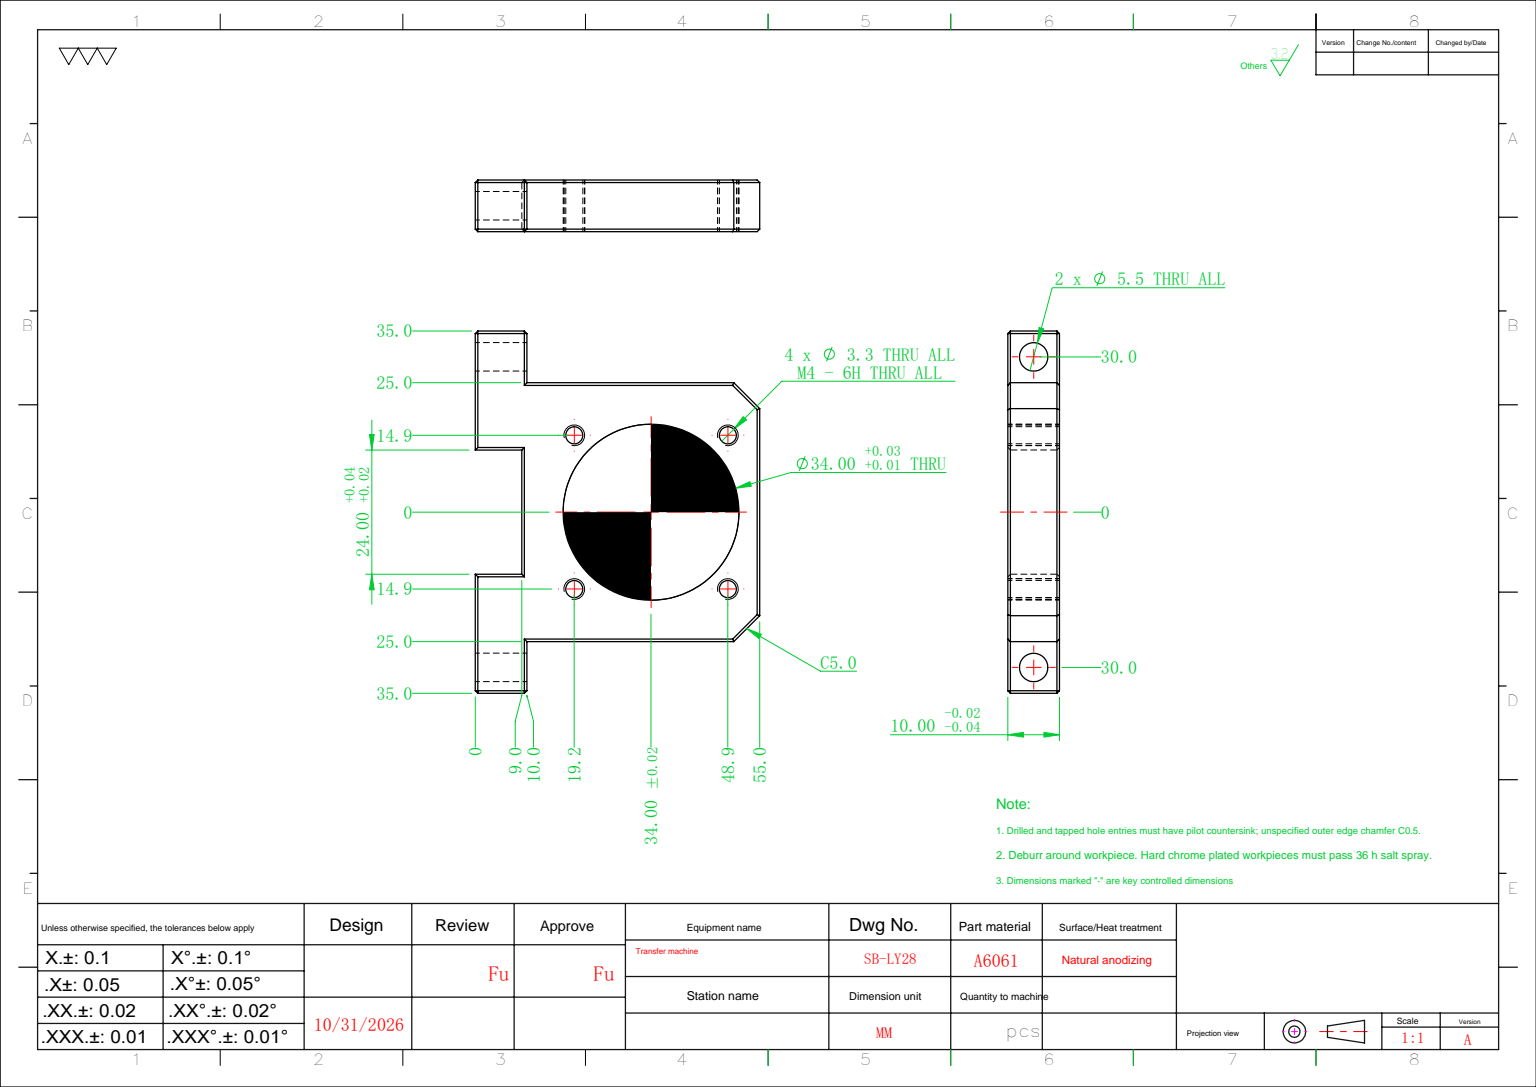
SolidWorks part; units mm, degrees
ref_plane "前视基准面" through (0, 0, 0) normal (0, 0, 1) x (1, 0, 0)
ref_plane "上视基准面" through (0, 0, 0) normal (0, 1, 0) x (1, 0, 0)
ref_plane "右视基准面" through (0, 0, 0) normal (1, 0, 0) x (0, 0, -1)
sketch "草图1" plane through (0, 0, 0) normal (0, 0, 1) x (1, 0, 0)
  line L1 (-35, -27.5) -> (35, -27.5)
  line L2 (-35, -27.5) -> (-35, 27.5)
  line L3 (-35, 27.5) -> (35, 27.5)
  line L4 (35, -27.5) -> (35, 27.5)
  line L5 (-35, -27.5) -> (35, 27.5) construction
  line L6 (-35, 27.5) -> (35, -27.5) construction
  point P0 (0, 0)
  dimension "D1" = 70
  dimension "D2" = 55
extrude "凸台-拉伸1" add sketch "草图1" along normal blind 10
sketch "草图2" plane through (0, 0, 10) normal (0, 0, 1) x (1, 0, 0)
  line L0 (0, 0) -> (0, -35.8295) construction
  line L1 (-35, -27.5) -> (-25, -27.5)
  line L2 (-35, -27.5) -> (-35, 17.5)
  line L3 (-35, 17.5) -> (-25, 17.5)
  line L4 (-25, -27.5) -> (-25, 17.5)
  line L5 (25, -27.5) -> (25, 17.5)
  line L6 (35, 17.5) -> (25, 17.5)
  line L7 (35, -27.5) -> (35, 17.5)
  line L8 (35, -27.5) -> (25, -27.5)
  line L9 (35, 27.5) -> (-35, 27.5) construction
  dimension "D1" = 10
  dimension "D2" = 10
extrude "切除-拉伸1" cut sketch "草图2" against normal through all
sketch "草图3" plane through (0, 0, 0) normal (0, 0, -1) x (-1, 0, 0)
  line L0 (0, 0) -> (0, -40.7468) construction
  line L1 (-35, 27.5) -> (35, 27.5) construction
  circle A0 centre (0, -6.5) radius 17
  dimension "D1" = 34
  dimension "D2" = 34
extrude "切除-拉伸2" cut sketch "草图3" against normal through all
hole_wizard "M4 螺纹孔2" positions "草图8" profile "草图9" tap size "M4" standard "ISO" end condition through all
sketch "草图8" plane through (0, 0, 10) normal (0, 0, 1) x (1, 0, 0)
  line L0 (0, -6.5) -> (0, -34.3856) construction
  line L3 (0, -6.5) -> (-29.4307, -6.5) construction
  point P0 (14.85, -21.35)
  point P2 (-14.85, -21.35)
  point P4 (-14.85, 8.35)
  point P6 (14.85, 8.35)
  dimension "D1" = 29.7
  dimension "D2" = 29.7
sketch "草图9" plane through (14.85, -21.35, 10) normal (1, 0, 0) x (0, -1, 0)
  line L0 (0, 0) -> (0, 10)
  line L1 (0, 10) -> (1.65, 10)
  line L2 (1.65, 10) -> (1.65, 0)
  line L5 (1.65, 0) -> (0, 0)
  line L11 (0, -6.35) -> (0, 107.95) construction
  dimension "通孔螺纹孔钻头直径" = 3.3
  dimension "通孔螺纹孔钻头深度" = 10
cosmetic thread "孔螺蚊线5" parameters "D2"=4
cosmetic thread "孔螺蚊线6" parameters "D2"=4
cosmetic thread "孔螺蚊线7" parameters "D2"=4
cosmetic thread "孔螺蚊线8" parameters "D2"=4
hole_wizard "Ø5.5 (5.5) 直径孔1" positions "草图10" profile "草图11" hole size "Ø5.5" standard "ISO" end condition through all
sketch "草图10" plane through (0, 17.5, 0) normal (0, -1, 0) x (-1, 0, 0)
  line L0 (35, -5) -> (-35, -5) construction
  line L1 (35, 0) -> (35, -10) construction
  line L2 (-35, 0) -> (-35, -10) construction
  line L4 (0, 0) -> (0, -15.7163) construction
  point P0 (-30, -5)
  point P2 (30, -5)
  dimension "D1" = 60
sketch "草图11" plane through (30, 17.5, 5) normal (1, 0, 0) x (0, 0, -1)
  line L0 (0, 0) -> (0, 10)
  line L1 (0, 10) -> (2.75, 10)
  line L2 (2.75, 10) -> (2.75, 0)
  line L5 (2.75, 0) -> (0, 0)
  line L11 (0, -6.35) -> (0, 107.95) construction
  dimension "通孔孔直径" = 5.5
  dimension "通孔孔深度" = 10
chamfer "倒角1" distance 5 angle 45 2 edges at (-25, -27.5, 5) (25, -27.5, 5)
sketch "草图12" plane through (0, 0, 10) normal (0, 0, 1) x (1, 0, 0)
  line L0 (35, 27.5) -> (-35, 27.5) construction
  line L1 (-12, 27.5) -> (12, 27.5)
  line L2 (-12, 27.5) -> (-12, 18.5)
  line L3 (-12, 18.5) -> (12, 18.5)
  line L4 (12, 27.5) -> (12, 18.5)
  line L5 (0, 0) -> (0, 36.1087) construction
  dimension "D1" = 24
  dimension "D2" = 9
extrude "切除-拉伸3" cut sketch "草图12" against normal through all
chamfer "倒角2" distance 0.5 angle 45 32 edges at (-23.5, 27.5, 0) (-30, 17.5, 0) (-25, -2.5, 0) (-22.5, -25, 0) (0, -27.5, 0) (22.5, -25, 0) (25, -2.5, 0) (30, 17.5, 0) (-12, 23, 0) (0, 18.5, 0) (12, 23, 0) (23.5, 27.5, 0) (12, 23, 10) (23.5, 27.5, 10) (0, 18.5, 10) (-12, 23, 10) (-23.5, 27.5, 10) (-35, 27.5, 5) (-35, 22.5, 10) (-35, 22.5, 0) (-35, 17.5, 5) (-30, 17.5, 10) (-25, -2.5, 10) (-22.5, -25, 10) (0, -27.5, 10) (22.5, -25, 10) (25, -2.5, 10) (30, 17.5, 10) (35, 27.5, 5) (35, 22.5, 0) (35, 17.5, 5) (35, 22.5, 10)
